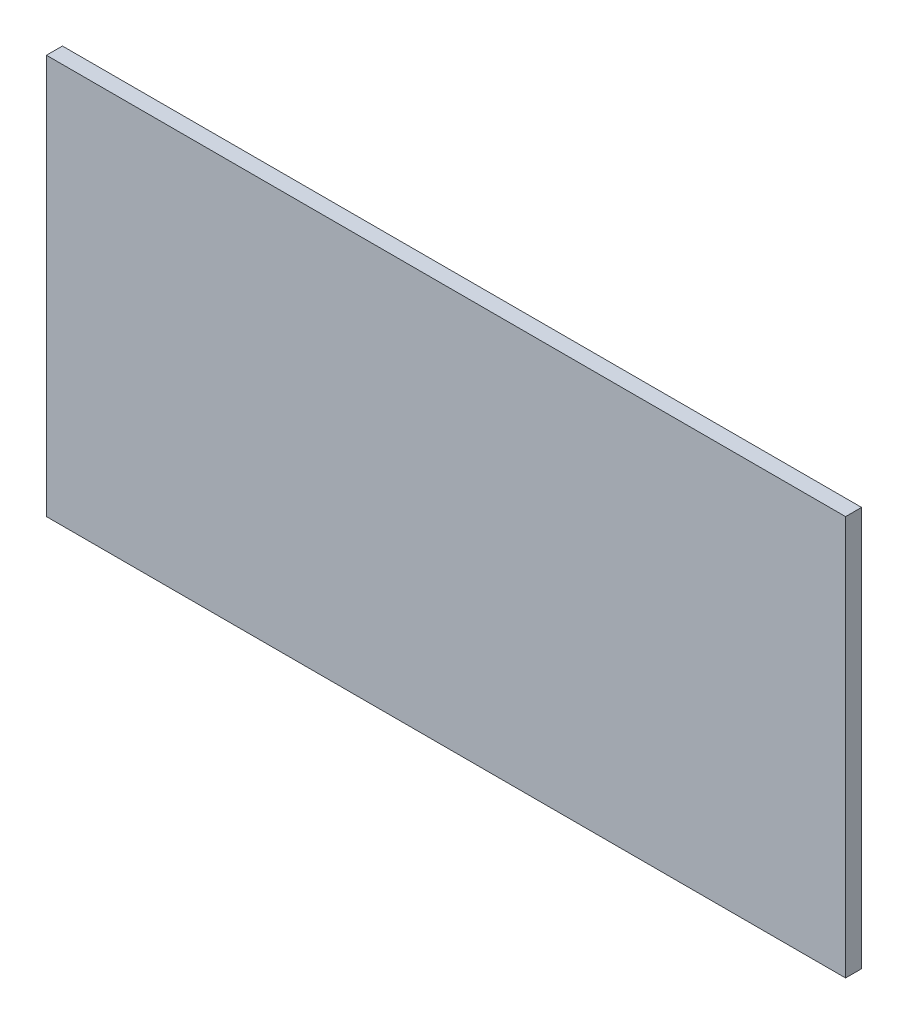
SolidWorks part; units mm, degrees
ref_plane "Front plane" through (0, 0, 0) normal (0, 0, 1) x (1, 0, 0)
ref_plane "Top plane" through (0, 0, 0) normal (0, 1, 0) x (1, 0, 0)
ref_plane "Right plane" through (0, 0, 0) normal (1, 0, 0) x (0, 0, -1)
sketch "Sketch1" plane through (0, 0, 0) normal (0, 0, 1) x (1, 0, 0)
  line L1 (-50, 25) -> (50, 25)
  line L2 (-50, 25) -> (-50, -25)
  line L3 (-50, -25) -> (50, -25)
  line L4 (50, 25) -> (50, -25)
  line L5 (-50, 25) -> (50, -25) construction
  line L6 (-50, -25) -> (50, 25) construction
  point P0 (0, 0)
  dimension "D1" = 100
  dimension "D2" = 50
extrude "Boss-Extrude1" add sketch "Sketch1" along normal blind 2
